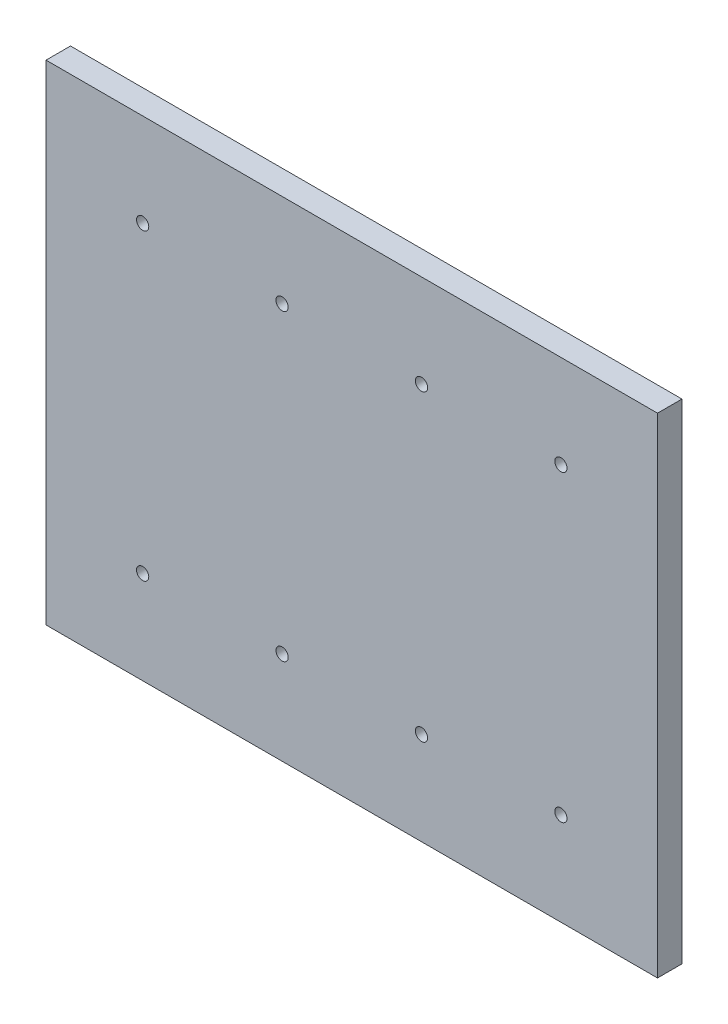
SolidWorks part; units mm, degrees
material "6061 合金"
ref_plane "Front Plane" through (0, 0, 0) normal (0, 0, 1) x (1, 0, 0)
ref_plane "Top Plane" through (0, 0, 0) normal (0, 1, 0) x (1, 0, 0)
ref_plane "Right Plane" through (0, 0, 0) normal (1, 0, 0) x (0, 0, -1)
sketch "Sketch1" plane through (0, 0, 0) normal (0, 0, 1) x (1, 0, 0)
  line L1 (-125, 100) -> (125, 100)
  line L2 (-125, 100) -> (-125, -100)
  line L3 (-125, -100) -> (125, -100)
  line L4 (125, 100) -> (125, -100)
  line L5 (-125, 100) -> (125, -100) construction
  line L6 (-125, -100) -> (125, 100) construction
  point P0 (0, 0)
  dimension "D1" = 250
  dimension "D2" = 200
extrude "Boss-Extrude1" add sketch "Sketch1" along normal blind 10
hole_wizard "M6 Tapped Hole1" positions "Sketch2" profile "Sketch3" tap size "M6" standard "ISO" end condition through all
sketch "Sketch2" plane through (0, 0, 10) normal (0, 0, 1) x (1, 0, 0)
  line L0 (0, 0) -> (49.6354, 0) construction
  point P0 (-85.5, 62)
  point P2 (-28.5, 62)
  point P4 (85.5, 62)
  point P7 (28.5, 62)
  point P15 (28.5, -62)
  point P16 (85.5, -62)
  point P17 (-28.5, -62)
  point P18 (-85.5, -62)
  dimension "D1" = 57
  dimension "D2" = 57
  dimension "D3" = 57
  dimension "D4" = 28.5
  dimension "D5" = 62
sketch "Sketch3" plane through (-85.5, 62, 10) normal (1, 0, 0) x (0, -1, 0)
  line L0 (0, 0) -> (0, 10)
  line L1 (0, 10) -> (2.5, 10)
  line L2 (2.5, 10) -> (2.5, 0)
  line L5 (2.5, 0) -> (0, 0)
  line L11 (0, -6.35) -> (0, 107.95) construction
  dimension "通孔螺纹孔钻头直径" = 5
  dimension "通孔螺纹孔钻头深度" = 10
cosmetic thread "Cosmetic Thread1"
cosmetic thread "Cosmetic Thread2"
cosmetic thread "Cosmetic Thread3"
cosmetic thread "Cosmetic Thread4"
cosmetic thread "Cosmetic Thread5"
cosmetic thread "Cosmetic Thread6"
cosmetic thread "Cosmetic Thread7"
cosmetic thread "Cosmetic Thread8"
